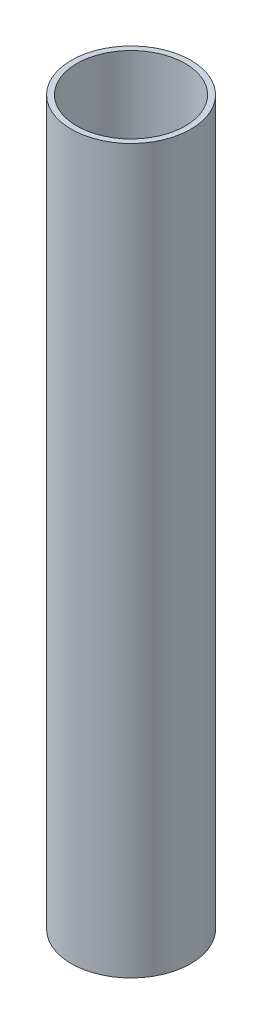
SolidWorks part; units mm, degrees
material "EVA"
ref_plane "前视基准面" through (0, 0, 0) normal (0, 0, 1) x (1, 0, 0)
ref_plane "上视基准面" through (0, 0, 0) normal (0, 1, 0) x (1, 0, 0)
ref_plane "右视基准面" through (0, 0, 0) normal (1, 0, 0) x (0, 0, -1)
sketch "草图1" plane through (0, 0, 0) normal (0, 1, 0) x (1, 0, 0)
  circle A0 centre (0, 0) radius 2.15
  dimension "D1" = 4.3
extrude "拉伸-薄壁1" add sketch "草图1" along normal blind 26 thin thin type one direction reverse wall 0.2
